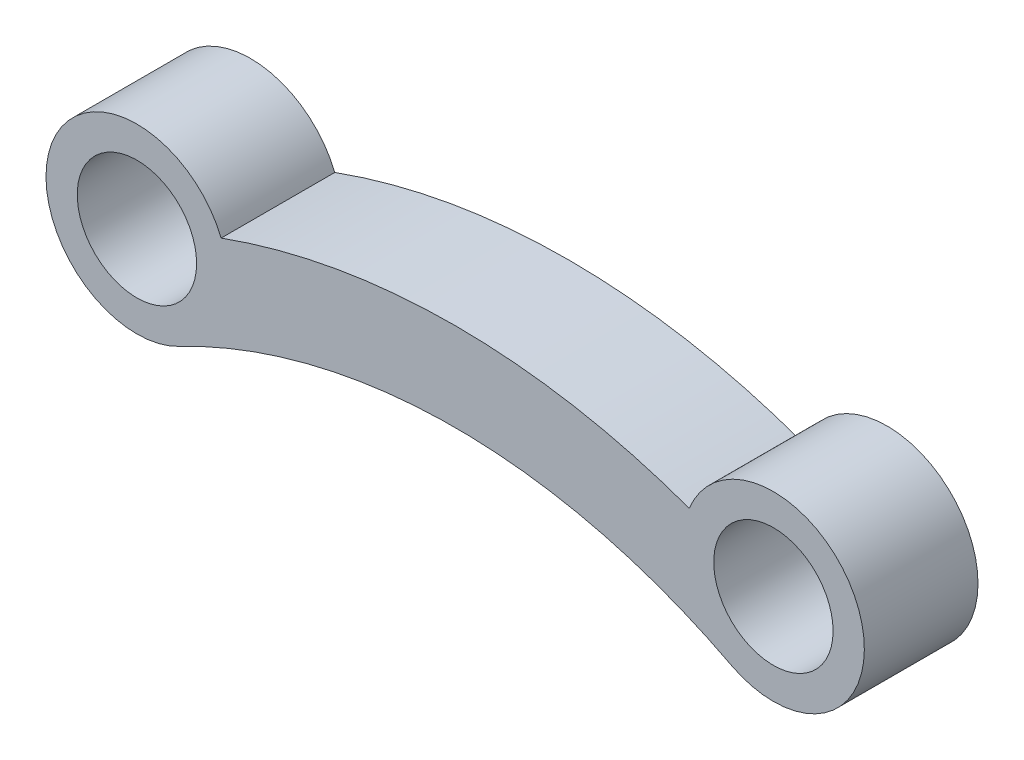
from build123d import *

# Parameters (mm, degrees)
BOSS_EXTRUDE1_DEPTH = 5
SKETCH2_R           = 1.5
CUT_EXTRUDE1_DEPTH  = 3
BOSS_EXTRUDE2_DEPTH = 5
SKETCH4_R           = 2.625
CUT_EXTRUDE2_DEPTH  = 34.097061453
CUT_EXTRUDE3_DEPTH  = 34.097061453
BOSS_EXTRUDE3_DEPTH = 5


with BuildPart() as part:
    # Sketch1 → Boss-Extrude1 (new body)
    with BuildSketch(Plane.XY):
        with BuildLine():
            ThreePointArc((-26.738194812, 2.158204732), (-30.234084304, -1.121992567), (-25.515357454, -0.276679267))
            ThreePointArc((-25.515357454, -0.276679267), (-19.880574881, 1.510931441), (-14, 2.115220905))
            ThreePointArc((-14, 2.115220905), (-8.119425119, 1.510931441), (-2.484642546, -0.276679267))
            ThreePointArc((-2.484642546, -0.276679267), (2.234084304, -1.121992567), (-1.261805188, 2.158204732))
            ThreePointArc((-1.261805188, 2.158204732), (-7.461545448, 4.366267273), (-14, 5.115220905))
            ThreePointArc((-14, 5.115220905), (-20.538454552, 4.366267273), (-26.738194812, 2.158204732))
        make_face()
    extrude(amount=BOSS_EXTRUDE1_DEPTH)

    # Sketch2 → Cut-Extrude1 (cut)
    with BuildSketch(Plane.XY.offset(5)):
        with Locations((-28, 0)):
            Circle(SKETCH2_R)
        Circle(SKETCH2_R)
    extrude(amount=-CUT_EXTRUDE1_DEPTH, mode=Mode.SUBTRACT)

    # Sketch3 → Boss-Extrude2 (add, through all)
    with BuildSketch(Plane.XY.offset(5)):
        with BuildLine():
            ThreePointArc((-27.059016708, 3.887743619), (-31.451726366, -2.021283032), (-24.149017572, -1.081635031))
            ThreePointArc((-24.149017572, -1.081635031), (-14, 0.848451211), (-3.850982428, -1.081635031))
            ThreePointArc((-3.850982428, -1.081635031), (3.451726366, -2.021283032), (-0.940983292, 3.887743619))
            ThreePointArc((-0.940983292, 3.887743619), (-13.167819997, 6.801577419), (-25.534946827, 4.556552431))
            ThreePointArc((-25.534946827, 4.556552431), (-26.301527828, 4.232507508), (-27.059016708, 3.887743619))
        make_face()
    extrude(amount=-BOSS_EXTRUDE2_DEPTH)

    # Sketch4 → Cut-Extrude2 (cut, through all)
    with BuildSketch(Plane.XY.offset(5)):
        with Locations((-28, 0)):
            Circle(SKETCH4_R)
        Circle(SKETCH4_R)
    extrude(amount=-CUT_EXTRUDE2_DEPTH, mode=Mode.SUBTRACT)

    # Sketch5 → Cut-Extrude3 (cut, through all)
    with BuildSketch(Plane.XY.offset(5)):
        with BuildLine():
            Line((-14.205977149, 10.740702715), (-0.940983292, 3.887743619))
            ThreePointArc((-0.940983292, 3.887743619), (-14, 6.812890489), (-27.059016708, 3.887743619))
            Line((-27.059016708, 3.887743619), (-14.205977149, 10.740702715))
        make_face()
        with BuildLine():
            ThreePointArc((-0.940983292, 3.887743619), (-14, 6.812890489), (-27.059016708, 3.887743619))
            ThreePointArc((-27.059016708, 3.887743619), (-25.390156506, 3.031289649), (-24.295234779, 1.50821572))
            ThreePointArc((-24.295234779, 1.50821572), (-14, 3.322200059), (-3.704765221, 1.50821572))
            ThreePointArc((-3.704765221, 1.50821572), (-2.609843494, 3.031289649), (-0.940983292, 3.887743619))
        make_face()
    extrude(amount=-CUT_EXTRUDE3_DEPTH, mode=Mode.SUBTRACT)

    # Sketch7 → Boss-Extrude3 (add, through all)
    with BuildSketch(Plane.XY.offset(5)):
        with BuildLine():
            Line((-26.14792778, -3.545395393), (-24.177787081, 0.278127161))
            Line((-24.177787081, 0.278127161), (-14.756553685, 2.142998553))
            Line((-14.756553685, 2.142998553), (-4.34233682, 0.278127161))
            Line((-4.34233682, 0.278127161), (-2.53651725, -2.31550038))
            Line((-2.53651725, -2.31550038), (-1.85207222, -3.545395393))
            ThreePointArc((-1.85207222, -3.545395393), (-14, -0.563598098), (-26.14792778, -3.545395393))
        make_face()
    extrude(amount=-BOSS_EXTRUDE3_DEPTH)


solid = part.part
